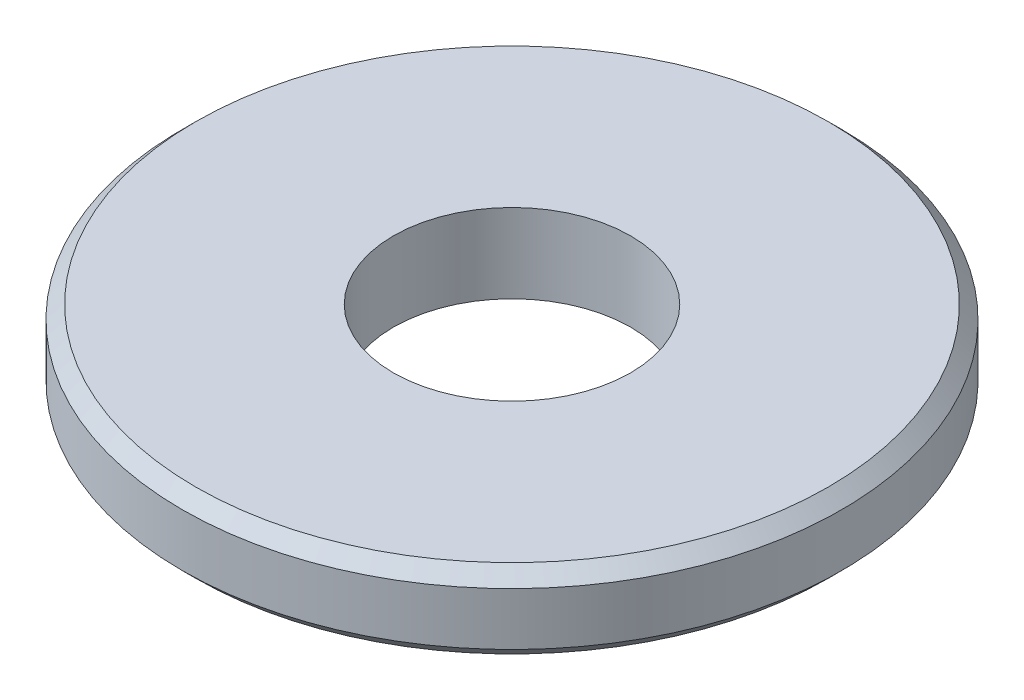
from build123d import *

# Parameters (mm, degrees)
SKETCH_1_R          = 12.5
EXTRUDE_1_DEPTH     = 3
SKETCH_2_R          = 4.5
CUT_EXTRUDE_1_DEPTH = 18.930421077
CHAMFER_1_SIZE      = 0.5


with BuildPart() as part:
    # 草图1 → 凸台-拉伸1 (new body)
    with BuildSketch(Plane(origin=(0, 0, 0), x_dir=(1, 0, 0), z_dir=(0, 1, 0))):
        with Locations(Location((0, 0, 0), (0, 0, 270))):
            Circle(SKETCH_1_R)
    extrude(amount=EXTRUDE_1_DEPTH)

    # 草图2 → 切除-拉伸1 (cut, through all)
    with BuildSketch(Plane(origin=(0, 3, 0), x_dir=(1, 0, 0), z_dir=(0, 1, 0))):
        with Locations(Location((0, 0, 0), (0, 0, 270))):
            Circle(SKETCH_2_R)
    extrude(amount=-CUT_EXTRUDE_1_DEPTH, mode=Mode.SUBTRACT)

    # 倒角1
    chamfer_1_edges = [part.edges().sort_by_distance(p)[0] for p in [
        (0, 0, -12.5),
        (0, 3, -12.5),
    ]]
    chamfer(chamfer_1_edges, length=CHAMFER_1_SIZE)


solid = part.part
